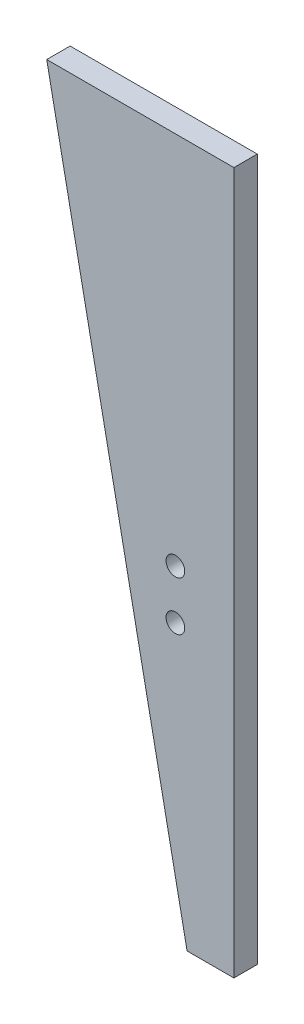
SolidWorks part; units mm, degrees
material "普通碳钢"
ref_plane "Front Plane" through (0, 0, 0) normal (0, 0, 1) x (1, 0, 0)
ref_plane "Top Plane" through (0, 0, 0) normal (0, 1, 0) x (1, 0, 0)
ref_plane "Right Plane" through (0, 0, 0) normal (1, 0, 0) x (0, 0, -1)
sketch "Sketch1" plane through (0, 0, 0) normal (0, 0, 1) x (1, 0, 0)
  line L0 (-80, 0) -> (0, 0)
  line L1 (0, 0) -> (0, -300)
  line L2 (0, -300) -> (-20, -300)
  line L3 (-20, -300) -> (-80, 0)
  dimension "D1" = 300
  dimension "D2" = 80
  dimension "D3" = 20
extrude "Extrude1" add sketch "Sketch1" along normal mid plane 10
sketch "Sketch2" plane through (0, 0, 5) normal (0, 0, 1) x (1, 0, 0)
  line L0 (0, -300) -> (0, 0) construction
  line L1 (0, 0) -> (-80, 0) construction
  circle A0 centre (-25, -160) radius 4
  circle A1 centre (-25, -181) radius 4
  dimension "D1" = 8
  dimension "D2" = 8
  dimension "D3" = 21
  dimension "D4" = 25
  dimension "D5" = 160
extrude "Extrude2" cut sketch "Sketch2" against normal blind 10
